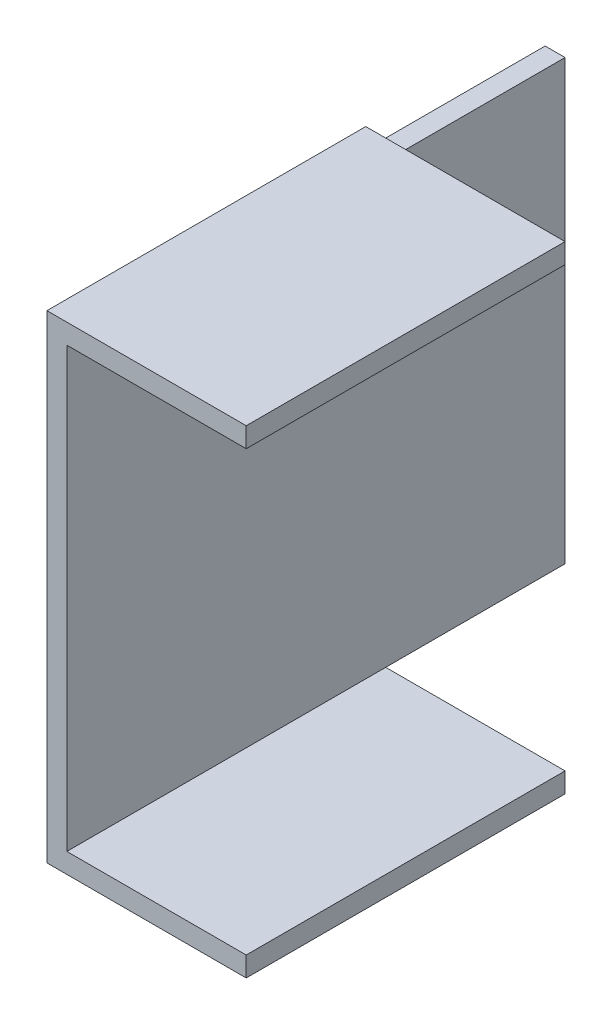
from build123d import *

# Parameters (mm, degrees)
EXTRUDE_1_DEPTH     = 150
SKETCH_2_W          = 50
SKETCH_2_H          = 5
CUT_EXTRUDE_1_DEPTH = 45
SKETCH_3_W          = 5
SKETCH_3_H          = 110
CUT_EXTRUDE_2_DEPTH = 25
CUT_EXTRUDE_3_DEPTH = 25
CUT_EXTRUDE_4_DEPTH = 25


with BuildPart() as part:
    # 草图1 → 凸台-拉伸1 (new body)
    with BuildSketch(Plane.XY):
        Polygon((0, 0), (0, 120), (50, 120), (50, 115), (5, 115), (5, 5), (50, 5), (50, 0), align=None)
    extrude(amount=-EXTRUDE_1_DEPTH)

    # 草图2 → 切除-拉伸1 (cut)
    with BuildSketch(Plane(origin=(0, 0, -150), x_dir=(-1, 0, 0), z_dir=(0, 0, -1))):
        with Locations((-25, 117.5)):
            Rectangle(SKETCH_2_W, SKETCH_2_H)
        with Locations((-25, 2.5)):
            Rectangle(SKETCH_2_W, SKETCH_2_H)
    extrude(amount=-CUT_EXTRUDE_1_DEPTH, mode=Mode.SUBTRACT)

    # 草图3 → 切除-拉伸2 (cut)
    with BuildSketch(Plane(origin=(0, 0, -150), x_dir=(-1, 0, 0), z_dir=(0, 0, -1))):
        with Locations((-2.5, 60)):
            Rectangle(SKETCH_3_W, SKETCH_3_H)
    extrude(amount=-CUT_EXTRUDE_2_DEPTH, mode=Mode.SUBTRACT)

    # 草图4 → 切除-拉伸3 (cut)
    with BuildSketch(Plane(origin=(0, 0, -105), x_dir=(-1, 0, 0), z_dir=(0, 0, -1))):
        Polygon((-50, 0), (0, 0), (0, 5), (-5, 5), (-50, 5), align=None)
    extrude(amount=-CUT_EXTRUDE_3_DEPTH, mode=Mode.SUBTRACT)

    # 草图5 → 切除-拉伸4 (cut)
    with BuildSketch(Plane(origin=(0, 0, -105), x_dir=(-1, 0, 0), z_dir=(0, 0, -1))):
        Polygon((-50, 120), (-50, 115), (-5, 115), (0, 115), (0, 120), align=None)
    extrude(amount=-CUT_EXTRUDE_4_DEPTH, mode=Mode.SUBTRACT)


solid = part.part
